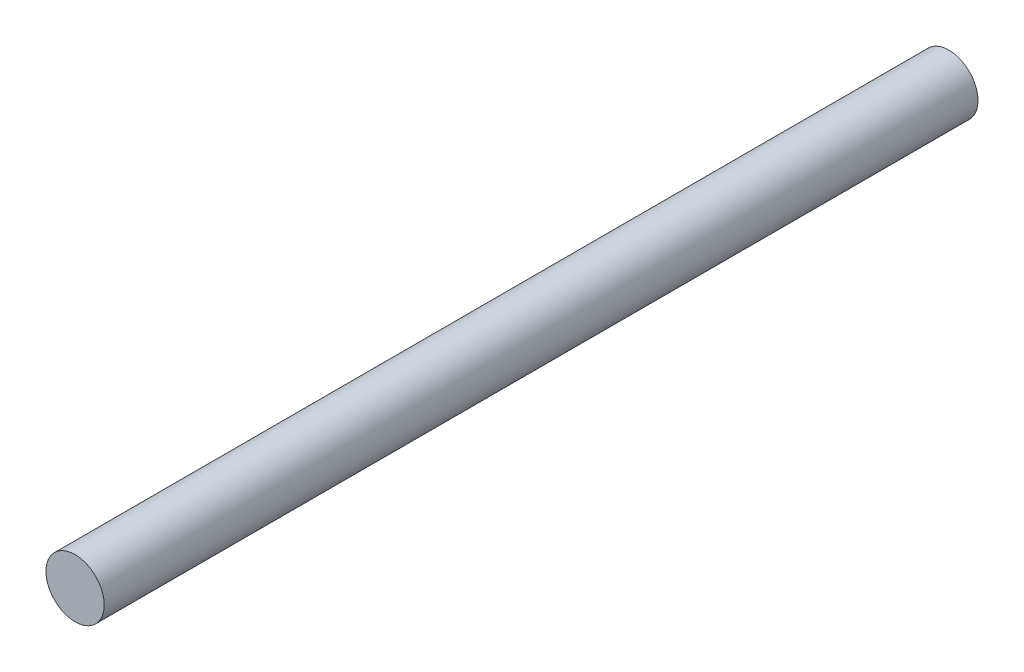
SolidWorks part; units mm, degrees
ref_plane "Front Plane" through (0, 0, 0) normal (0, 0, 1) x (1, 0, 0)
ref_plane "Top Plane" through (0, 0, 0) normal (0, 1, 0) x (1, 0, 0)
ref_plane "Right Plane" through (0, 0, 0) normal (1, 0, 0) x (0, 0, -1)
sketch "Sketch1" plane through (0, 0, 0) normal (0, 0, 1) x (1, 0, 0)
  circle A0 centre (0, 0) radius 1
  dimension "D1" = 2
extrude "Boss-Extrude1" add sketch "Sketch1" along normal blind 30
